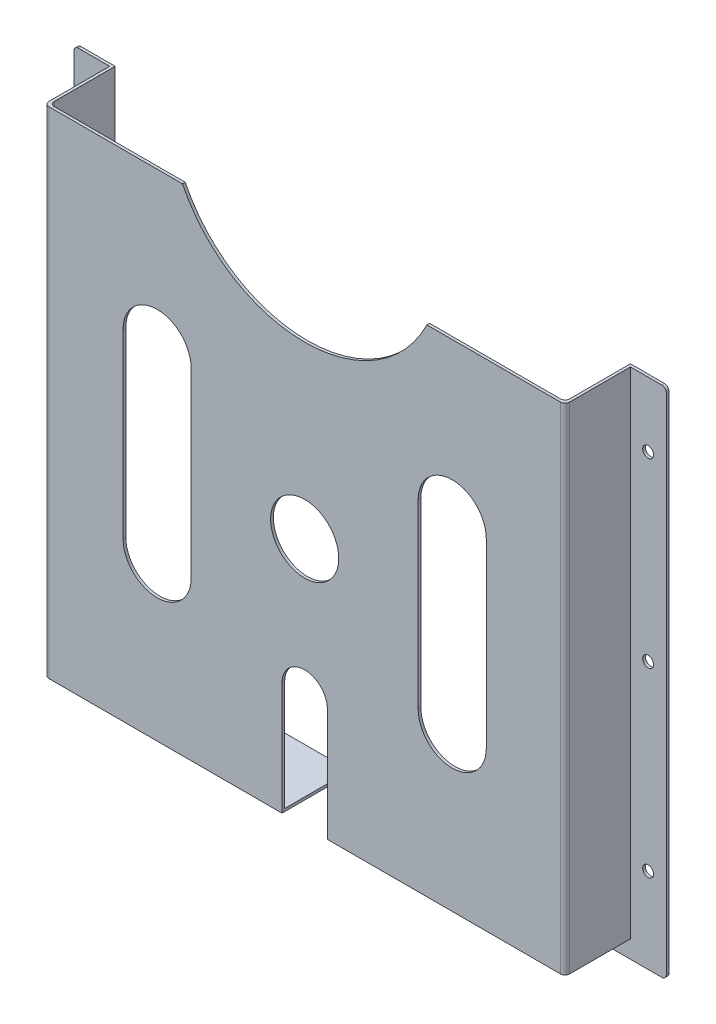
from build123d import *

# Parameters (mm, degrees)
SKETCH1_W            = 227
SKETCH1_H            = 217
BOSS_EXTRUDE1_DEPTH  = 1.2
SKETCH21_W           = 229.4
SKETCH21_H           = 219.4
SKETCH21_W_2         = 227
SKETCH21_H_2         = 217
BOSS_EXTRUDE2_DEPTH  = 30
SKETCH22_W           = 261
SKETCH22_H           = 235
SKETCH22_W_2         = 227
SKETCH22_H_2         = 217
BOSS_EXTRUDE3_DEPTH  = 1.2
SKETCH23_W           = 261
SKETCH23_H           = 30
CUT_EXTRUDE1_DEPTH   = 9
CUT_EXTRUDE2_START   = -28.8
SKETCH24_R           = 15
SKETCH24_R_2         = 60
CUT_EXTRUDE2_DEPTH   = 28.8
FILLET1_R            = 2
FILLET2_R            = 2
M4_CLEARANCE_HOLE1_D = 4.8


with BuildPart() as part:
    # Sketch1 → Boss-Extrude1 (new body)
    with BuildSketch(Plane.XY):
        Rectangle(SKETCH1_W, SKETCH1_H)
    extrude(amount=BOSS_EXTRUDE1_DEPTH)

    # Sketch21 → Boss-Extrude2 (add)
    with BuildSketch(Plane.XY.offset(1.2)):
        Rectangle(SKETCH21_W, SKETCH21_H)
        Rectangle(SKETCH21_W_2, SKETCH21_H_2, mode=Mode.SUBTRACT)
    extrude(amount=-BOSS_EXTRUDE2_DEPTH)

    # Sketch22 → Boss-Extrude3 (add)
    with BuildSketch(Plane(origin=(0, 0, -28.8), x_dir=(-1, 0, 0), z_dir=(0, 0, -1))):
        Rectangle(SKETCH22_W, SKETCH22_H)
        Rectangle(SKETCH22_W_2, SKETCH22_H_2, mode=Mode.SUBTRACT)
    extrude(amount=-BOSS_EXTRUDE3_DEPTH)

    # Sketch23 → Cut-Extrude1 (cut)
    with BuildSketch(Plane(origin=(0, 117.5, 0), x_dir=(1, 0, 0), z_dir=(0, 1, 0))):
        with Locations((0, 13.8)):
            Rectangle(SKETCH23_W, SKETCH23_H)
    extrude(amount=-CUT_EXTRUDE1_DEPTH, mode=Mode.SUBTRACT)

    # Sketch24 → Cut-Extrude2 (cut)
    with BuildSketch(Plane.XY.offset(1.2).offset(CUT_EXTRUDE2_START)):
        Circle(SKETCH24_R)
        with Locations((0, 135)):
            Circle(SKETCH24_R_2)
        with BuildLine():
            Line((-80, -40), (-80, 40))
            ThreePointArc((-80, 40), (-65, 55), (-50, 40))
            Line((-50, 40), (-50, -40))
            ThreePointArc((-50, -40), (-65, -55), (-80, -40))
        make_face()
        with BuildLine():
            Line((80, -40), (80, 40))
            ThreePointArc((80, 40), (65, 55), (50, 40))
            Line((50, 40), (50, -40))
            ThreePointArc((50, -40), (65, -55), (80, -40))
        make_face()
        with BuildLine():
            Line((10, -60), (10, -120))
            ThreePointArc((10, -120), (0, -130), (-10, -120))
            Line((-10, -120), (-10, -60))
            ThreePointArc((-10, -60), (0, -50), (10, -60))
        make_face()
    extrude(amount=CUT_EXTRUDE2_DEPTH, mode=Mode.SUBTRACT)

    # Fillet1
    fillet1_edges = [part.edges().sort_by_distance(p)[0] for p in [
        (114.7, -0.6, 1.2),
        (-113.5, 0, 0),
        (113.5, 0, 0),
        (-114.7, -0.6, 1.2),
    ]]
    fillet(fillet1_edges, radius=FILLET1_R)

    # Fillet2
    fillet2_edges = [part.edges().sort_by_distance(p)[0] for p in [
        (-130.5, -117.5, -28.2),
        (130.5, -117.5, -28.2),
        (130.5, 108.5, -28.2),
        (-130.5, 108.5, -28.2),
    ]]
    fillet(fillet2_edges, radius=FILLET2_R)

    # M4 Clearance Hole1 (through all)
    with Locations(Plane.XY.offset(-27.6)):
        with Locations((-122.5, 80)):
            m4_clearance_hole1 = Hole(M4_CLEARANCE_HOLE1_D / 2)

    # Sketch pattern1: M4 Clearance Hole1 at 5 more places
    with Locations((0, -80, 0), (0, -160, 0), (245, -160, 0), (245, -80, 0), (245, 0, 0)):
        add(m4_clearance_hole1, mode=Mode.SUBTRACT)


solid = part.part
